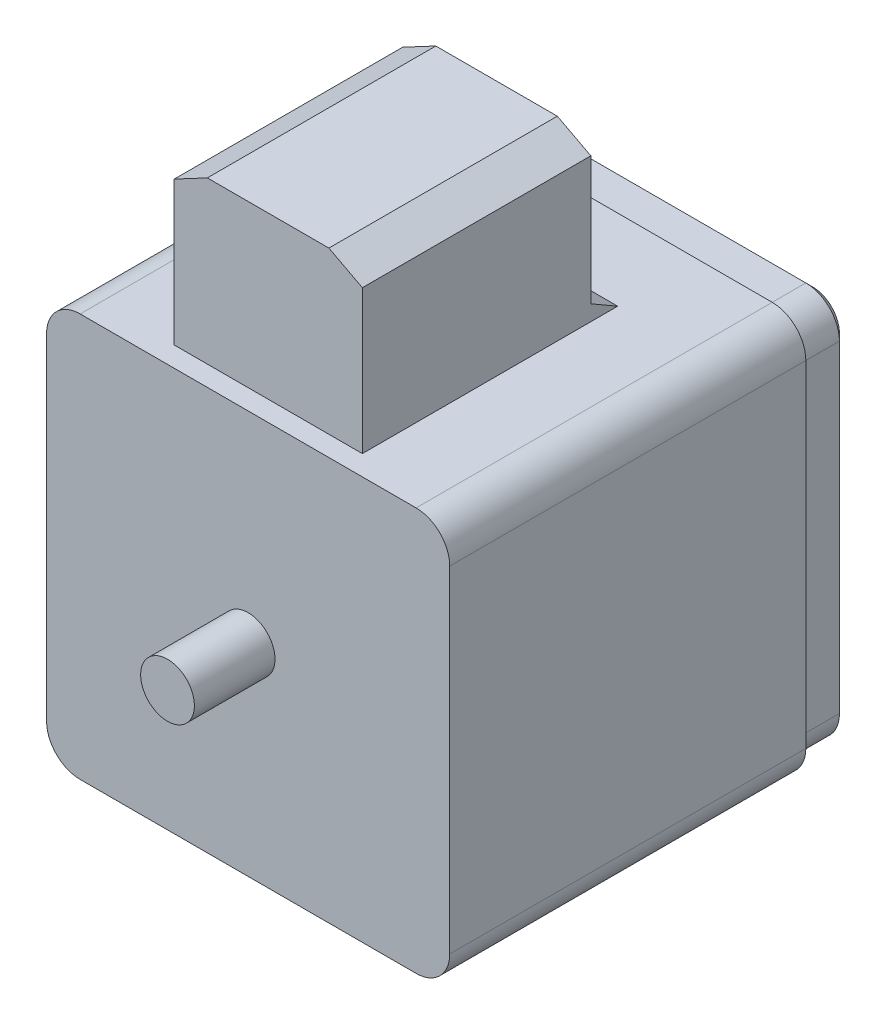
from build123d import *

# Parameters (mm, degrees)
SKETCH_1_W          = 60
SKETCH_1_H          = 60
EXTRUDE_1_DEPTH     = 60
SKETCH_2_R          = 4
EXTRUDE_2_DEPTH     = 12
SKETCH_3_W          = 60
SKETCH_3_H          = 60
SKETCH_3_W_2        = 58
SKETCH_3_H_2        = 58
CUT_EXTRUDE_1_DEPTH = 7
FILLET_1_R          = 5
CHAMFER_1_SIZE      = 1
FILLET_2_R          = 5
SKETCH_5_W          = 28
SKETCH_5_H          = 38
EXTRUDE_3_DEPTH     = 24
SKETCH_6_W          = 44.228024493
SKETCH_6_H          = 29.890039758
SKETCH_6_R          = 7.083561646
CUT_EXTRUDE_2_DEPTH = 4
CUT_EXTRUDE_2_DRAFT = -30
CUT_EXTRUDE_3_DEPTH = 79.847954951


with BuildPart() as part:
    # 草图1 → 凸台-拉伸1 (new body)
    with BuildSketch(Plane.XY):
        Rectangle(SKETCH_1_W, SKETCH_1_H)
    extrude(amount=EXTRUDE_1_DEPTH)

    # 草图2 → 凸台-拉伸2 (add)
    with BuildSketch(Plane.XY.offset(60)):
        with Locations(Location((0, 0, 0), (0, 0, 180))):
            Circle(SKETCH_2_R)
    extrude(amount=EXTRUDE_2_DEPTH)

    # 草图3 → 切除-拉伸1 (cut)
    with BuildSketch(Plane(origin=(0, 0, 0), x_dir=(-1, 0, 0), z_dir=(0, 0, -1))):
        Rectangle(SKETCH_3_W, SKETCH_3_H)
        Rectangle(SKETCH_3_W_2, SKETCH_3_H_2, mode=Mode.SUBTRACT)
    extrude(amount=-CUT_EXTRUDE_1_DEPTH, mode=Mode.SUBTRACT)

    # 圆角1
    fillet_1_edges = [part.edges().sort_by_distance(p)[0] for p in [
        (-29, -29, 3.5),
        (29, -29, 3.5),
        (29, 29, 3.5),
        (-29, 29, 3.5),
    ]]
    fillet(fillet_1_edges, radius=FILLET_1_R)

    # 倒角1
    chamfer_1_edges = [part.edges().sort_by_distance(p)[0] for p in [
        (-29, 0, 0),
        (0, -29, 0),
        (0, 29, 0),
        (29, 0, 0),
        (27.535533906, 27.535533906, 0),
        (27.535533906, -27.535533906, 0),
        (-27.535533906, -27.535533906, 0),
        (-27.535533906, 27.535533906, 0),
    ]]
    chamfer(chamfer_1_edges, length=CHAMFER_1_SIZE)

    # 圆角2
    fillet_2_edges = [part.edges().sort_by_distance(p)[0] for p in [
        (30, -30, 33.5),
        (-30, -30, 33.5),
        (-30, 30, 33.5),
        (30, 30, 33.5),
    ]]
    fillet(fillet_2_edges, radius=FILLET_2_R)

    # 草图5 → 凸台-拉伸3 (add)
    with BuildSketch(Plane(origin=(0, 30, 0), x_dir=(1, 0, 0), z_dir=(0, 1, 0))):
        with Locations((0, -38)):
            Rectangle(SKETCH_5_W, SKETCH_5_H)
    extrude(amount=EXTRUDE_3_DEPTH)


with BuildPart() as cut_extrude_2_tool:
    # 草图6 → 切除-拉伸2 (with draft: the straight prism first)
    with BuildSketch(Plane(origin=(0, 0, 19), x_dir=(-1, 0, 0), z_dir=(0, 0, -1))):
        with Locations((-0.478057726, 44.945019879)):
            Rectangle(SKETCH_6_W, SKETCH_6_H)
        with Locations((0, 42)):
            Circle(SKETCH_6_R, mode=Mode.SUBTRACT)
    extrude(amount=-CUT_EXTRUDE_2_DEPTH)
    # 切除-拉伸2: the draft: its side faces are tilted about the plane it starts from
    cut_extrude_2_sides = [cut_extrude_2_tool.faces().sort_by_distance(p)[0] for p in [
        (22.592069973, 44.945019879, 21),
        (0.478057727, 30, 21),
        (-21.63595452, 44.945019879, 21),
        (0.478057727, 59.890039758, 21),
        (7.083561646, 42, 21),
    ]]
    draft(cut_extrude_2_sides, Plane(origin=(0, 0, 19), x_dir=(-1, 0, 0), z_dir=(0, 0, -1)), CUT_EXTRUDE_2_DRAFT)


with BuildPart() as part_1:
    add(part.part)

    # 切除-拉伸2: cut by cut_extrude_2_tool
    add(cut_extrude_2_tool.part, mode=Mode.SUBTRACT)

    # 草图7 → 切除-拉伸3 (cut, through all)
    with BuildSketch(Plane(origin=(0, 0, 23), x_dir=(-1, 0, 0), z_dir=(0, 0, -1))):
        Polygon((-14, 51.383198576), (-9.015728145, 54), (9.073415265, 54), (14, 51.383198576), (16.492135927, 52.691599288), (15.246067964, 56.551525264), (-18.004122386, 56.551525264), align=None)
    extrude(amount=-CUT_EXTRUDE_3_DEPTH, mode=Mode.SUBTRACT)


solid = part_1.part
